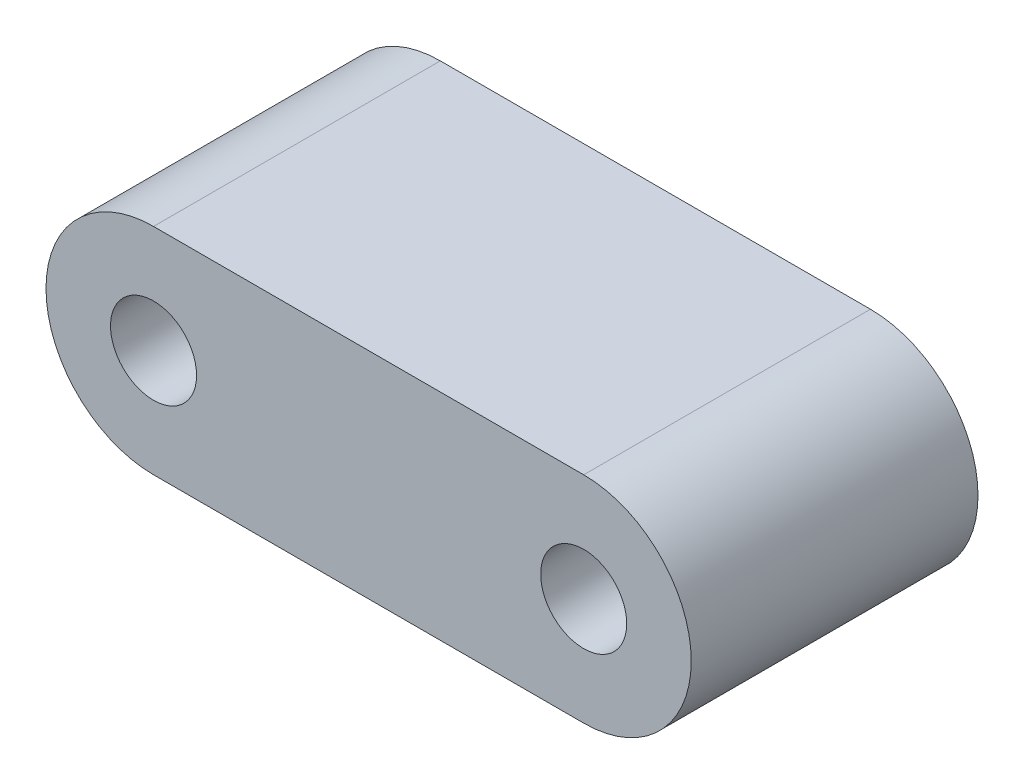
SolidWorks part; units mm, degrees
ref_plane "Front Plane" through (0, 0, 0) normal (0, 0, 1) x (1, 0, 0)
ref_plane "Top Plane" through (0, 0, 0) normal (0, 1, 0) x (1, 0, 0)
ref_plane "Right Plane" through (0, 0, 0) normal (1, 0, 0) x (0, 0, -1)
sketch "Sketch1" plane through (0, 0, 0) normal (0, 0, 1) x (1, 0, 0)
  line L0 (0, 0) -> (30, 0) construction
  line L1 (0, 7.5) -> (30, 7.5)
  line L2 (0, -7.5) -> (30, -7.5)
  arc A0 (0, 7.5) -> (0, -7.5) centre (0, 0) ccw
  arc A1 (30, -7.5) -> (30, 7.5) centre (30, 0) ccw
  circle A2 centre (0, 0) radius 3
  circle A3 centre (30, 0) radius 3
  point P3 (15, 0)
  dimension "D3" = 6
  dimension "D1" = 15
  dimension "D2" = 30
extrude "Boss-Extrude1" add sketch "Sketch1" along normal blind 20
